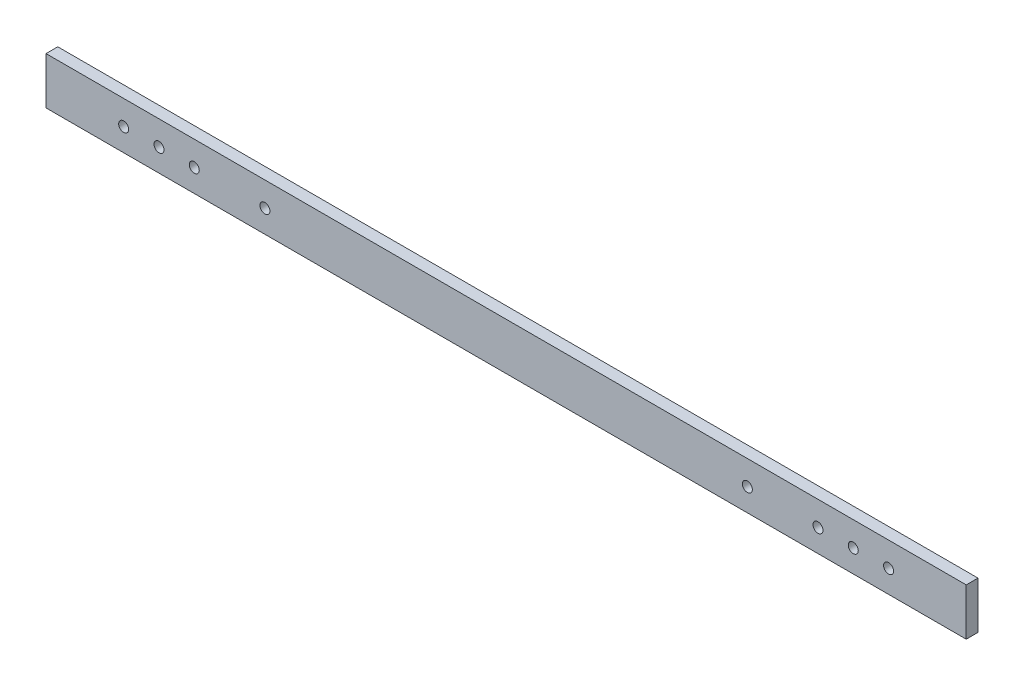
from build123d import *

# Parameters (mm, degrees)
SKETCH1_W              = 782
SKETCH1_H              = 40
BOSS_EXTRUDE1_DEPTH    = 10
M10_TAPPED_HOLE3_D     = 8.5
M10_TAPPED_HOLE3_DEPTH = 24.5
M10_TAPPED_HOLE3_TIP   = 2.553657631


with BuildPart() as part:
    # Sketch1 → Boss-Extrude1 (new body)
    with BuildSketch(Plane.XY):
        Rectangle(SKETCH1_W, SKETCH1_H)
    extrude(amount=BOSS_EXTRUDE1_DEPTH)

    # M10 Tapped Hole3
    with Locations(Plane.XY.offset(10)):
        with Locations((-325, -0.78), (-295, -0.78), (-265, -0.78), (-205, -0.78), (205, -0.78), (265, -0.78), (295, -0.78), (325, -0.78)):
            Hole(M10_TAPPED_HOLE3_D / 2, depth=M10_TAPPED_HOLE3_DEPTH)
            with Locations((0, 0, -(M10_TAPPED_HOLE3_DEPTH + M10_TAPPED_HOLE3_TIP / 2))):  # 118° drill point
                Cone(0, M10_TAPPED_HOLE3_D / 2, M10_TAPPED_HOLE3_TIP, mode=Mode.SUBTRACT)


solid = part.part
